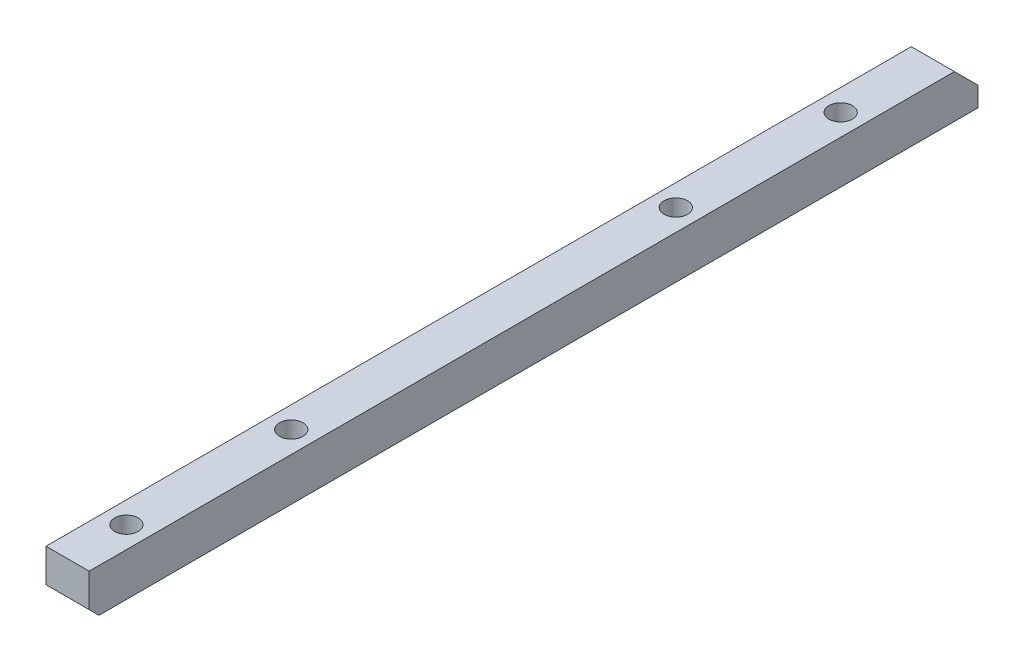
SolidWorks part; units mm, degrees
material "SS400B"
ref_plane "Front Plane" through (0, 0, 0) normal (0, 0, 1) x (1, 0, 0)
ref_plane "Top Plane" through (0, 0, 0) normal (0, 1, 0) x (1, 0, 0)
ref_plane "Right Plane" through (0, 0, 0) normal (1, 0, 0) x (0, 0, -1)
sketch "Sketch1" plane through (0, 0, 0) normal (0, 0, 1) x (1, 0, 0)
  line L1 (-11, 11) -> (11, 11)
  line L2 (-11, 11) -> (-11, -11)
  line L3 (-11, -11) -> (11, -11)
  line L4 (11, 11) -> (11, -11)
  line L5 (-11, 11) -> (11, -11) construction
  line L6 (-11, -11) -> (11, 11) construction
  point P0 (0, 0)
  dimension "D1" = 22
  dimension "D2" = 22
extrude "Boss-Extrude1" add sketch "Sketch1" along normal mid plane 453
sketch "Sketch2" plane through (0, 11, 0) normal (0, 1, 0) x (1, 0, 0)
  line L0 (11, -226.5) -> (-11, -226.5) construction
  circle A0 centre (0, -196.5) radius 6
  circle A1 centre (0, -112.5) radius 6
  circle A2 centre (0, 83.5) radius 6
  circle A3 centre (0, 167.5) radius 6
  dimension "D1" = 12
  dimension "D3" = 84
  dimension "D4" = 280
  dimension "D5" = 364
  dimension "D2" = 30
extrude "Cut-Extrude1" cut sketch "Sketch2" against normal through all
chamfer "Chamfer1" distance 5 angle 45 1 edges at (0, -11, 226.5)
chamfer "Chamfer2" distance 12 angle 45 1 edges at (0, 11, -226.5)
